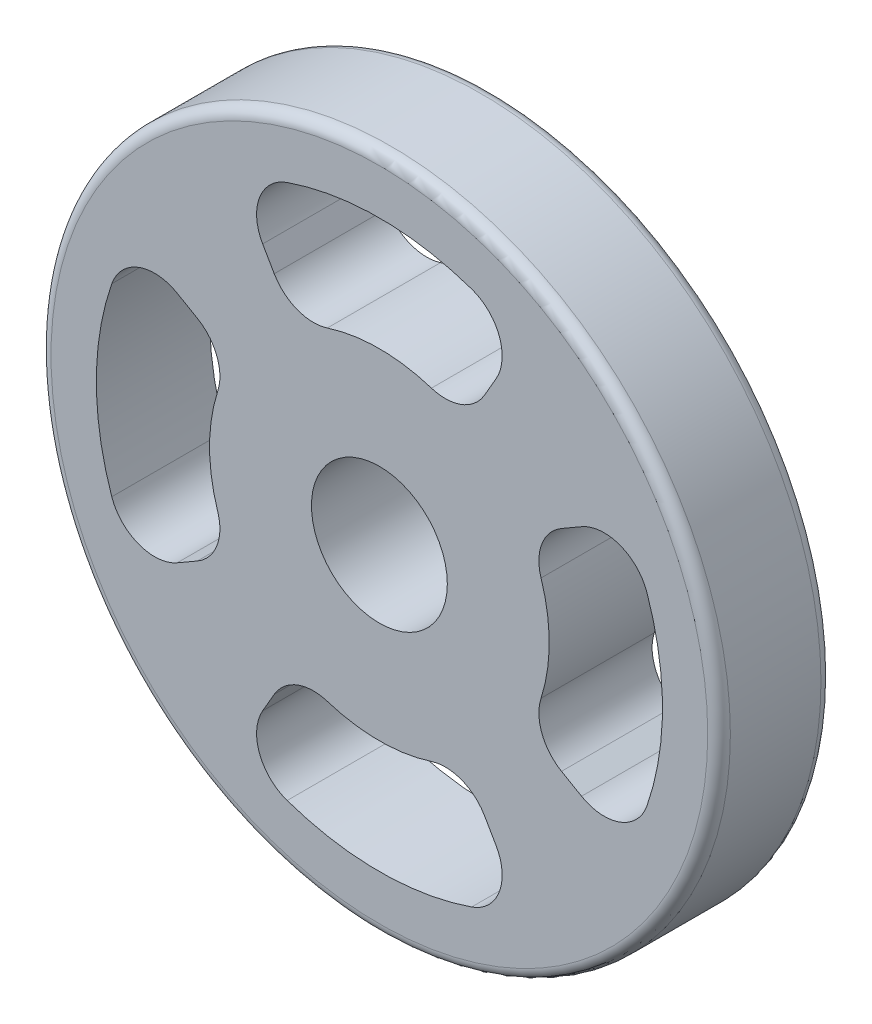
from build123d import *

# Parameters (mm, degrees)
SKETCH1_R           = 15
SKETCH1_R_2         = 3
BOSS_EXTRUDE1_DEPTH = 5
CUT_EXTRUDE1_DEPTH  = 5
FILLET1_R           = 0.5


with BuildPart() as part:
    # Sketch1 → Boss-Extrude1 (new body)
    with BuildSketch(Plane.XY):
        Circle(SKETCH1_R)
        Circle(SKETCH1_R_2, mode=Mode.SUBTRACT)
    extrude(amount=BOSS_EXTRUDE1_DEPTH)

    # Sketch2 → Cut-Extrude1 (cut)
    with BuildSketch(Plane.XY.offset(5)):
        with BuildLine():
            Line((-5.153882032, 8.926785536), (-4.643543905, 8.042853971))
            ThreePointArc((-4.643543905, 8.042853971), (-3.630724563, 7.176652991), (-2.298547182, 7.13909524))
            ThreePointArc((-2.298547182, 7.13909524), (0, 7.5), (2.298547182, 7.13909524))
            ThreePointArc((2.298547182, 7.13909524), (3.630724563, 7.176652991), (4.643543905, 8.042853971))
            Line((4.643543905, 8.042853971), (5.153882032, 8.926785536))
            ThreePointArc((5.153882032, 8.926785536), (5.295294304, 10.626882735), (4.073608601, 11.817601828))
            ThreePointArc((4.073608601, 11.817601828), (0, 12.5), (-4.073608601, 11.817601828))
            ThreePointArc((-4.073608601, 11.817601828), (-5.295294304, 10.626882735), (-5.153882032, 8.926785536))
        make_face()
        with BuildLine():
            Line((8.926785536, 5.153882032), (8.042853971, 4.643543905))
            ThreePointArc((8.042853971, 4.643543905), (7.176652991, 3.630724563), (7.13909524, 2.298547182))
            ThreePointArc((7.13909524, 2.298547182), (7.5, 0), (7.13909524, -2.298547182))
            ThreePointArc((7.13909524, -2.298547182), (7.176652991, -3.630724563), (8.042853971, -4.643543905))
            Line((8.042853971, -4.643543905), (8.926785536, -5.153882032))
            ThreePointArc((8.926785536, -5.153882032), (10.626882735, -5.295294304), (11.817601828, -4.073608601))
            ThreePointArc((11.817601828, -4.073608601), (12.5, 0), (11.817601828, 4.073608601))
            ThreePointArc((11.817601828, 4.073608601), (10.626882735, 5.295294304), (8.926785536, 5.153882032))
        make_face()
        with BuildLine():
            Line((5.153882032, -8.926785536), (4.643543905, -8.042853971))
            ThreePointArc((4.643543905, -8.042853971), (3.630724563, -7.176652991), (2.298547182, -7.13909524))
            ThreePointArc((2.298547182, -7.13909524), (0, -7.5), (-2.298547182, -7.13909524))
            ThreePointArc((-2.298547182, -7.13909524), (-3.630724563, -7.176652991), (-4.643543905, -8.042853971))
            Line((-4.643543905, -8.042853971), (-5.153882032, -8.926785536))
            ThreePointArc((-5.153882032, -8.926785536), (-5.295294304, -10.626882735), (-4.073608601, -11.817601828))
            ThreePointArc((-4.073608601, -11.817601828), (0, -12.5), (4.073608601, -11.817601828))
            ThreePointArc((4.073608601, -11.817601828), (5.295294304, -10.626882735), (5.153882032, -8.926785536))
        make_face()
        with BuildLine():
            Line((-8.926785536, -5.153882032), (-8.042853971, -4.643543905))
            ThreePointArc((-8.042853971, -4.643543905), (-7.176652991, -3.630724563), (-7.13909524, -2.298547182))
            ThreePointArc((-7.13909524, -2.298547182), (-7.5, 0), (-7.13909524, 2.298547182))
            ThreePointArc((-7.13909524, 2.298547182), (-7.176652991, 3.630724563), (-8.042853971, 4.643543905))
            Line((-8.042853971, 4.643543905), (-8.926785536, 5.153882032))
            ThreePointArc((-8.926785536, 5.153882032), (-10.626882735, 5.295294304), (-11.817601828, 4.073608601))
            ThreePointArc((-11.817601828, 4.073608601), (-12.5, 0), (-11.817601828, -4.073608601))
            ThreePointArc((-11.817601828, -4.073608601), (-10.626882735, -5.295294304), (-8.926785536, -5.153882032))
        make_face()
    extrude(amount=-CUT_EXTRUDE1_DEPTH, mode=Mode.SUBTRACT)

    # Fillet1
    fillet1_edges = [part.edges().sort_by_distance(p)[0] for p in [
        (-15, 0, 0),
        (-15, 0, 5),
    ]]
    fillet(fillet1_edges, radius=FILLET1_R)


solid = part.part
